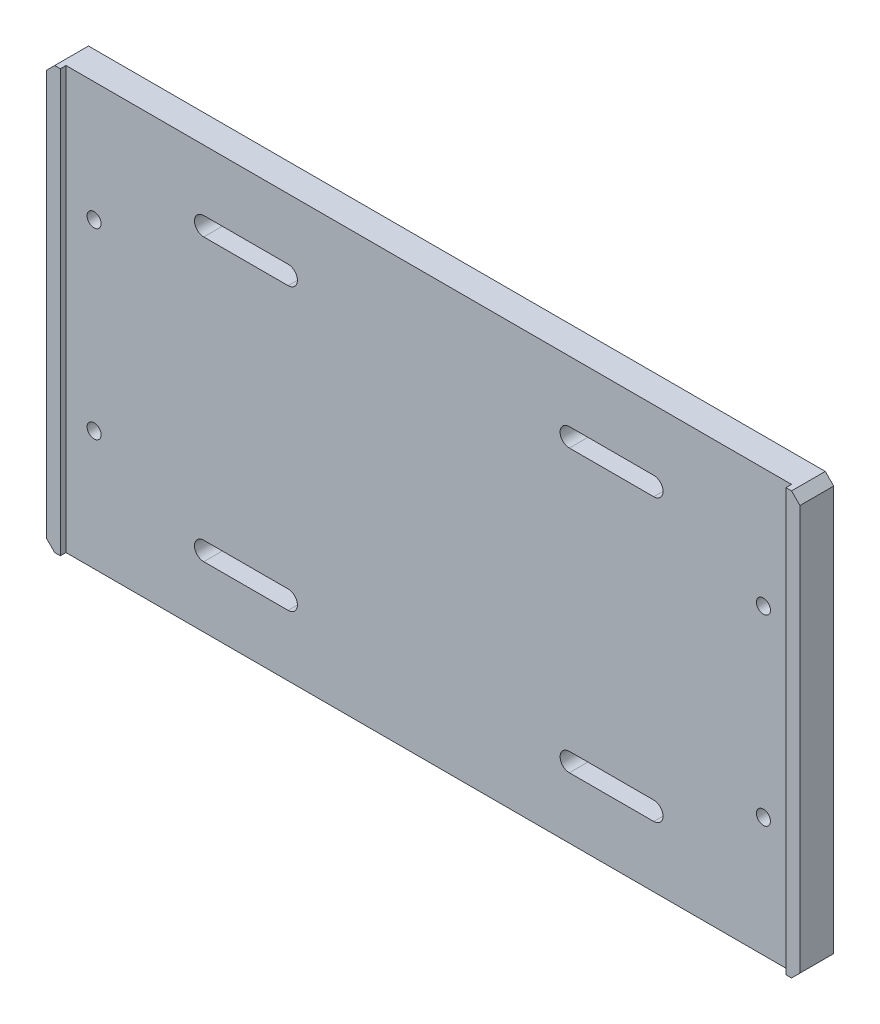
SolidWorks part; units mm, degrees
ref_plane "前视基准面" through (0, 0, 0) normal (0, 0, 1) x (1, 0, 0)
ref_plane "上视基准面" through (0, 0, 0) normal (0, 1, 0) x (1, 0, 0)
ref_plane "右视基准面" through (0, 0, 0) normal (1, 0, 0) x (0, 0, -1)
sketch "草图1" plane through (0, 0, 0) normal (0, 0, 1) x (1, 0, 0)
  line L1 (-134, -75) -> (134, -75)
  line L2 (-134, -75) -> (-134, 75)
  line L3 (-134, 75) -> (134, 75)
  line L4 (134, -75) -> (134, 75)
  line L5 (-134, -75) -> (134, 75) construction
  line L6 (-134, 75) -> (134, -75) construction
  point P0 (0, 0)
  dimension "D1" = 268
  dimension "D2" = 150
extrude "凸台-拉伸1" add sketch "草图1" along normal blind 12
sketch "草图2" plane through (0, 0, 12) normal (0, 0, 1) x (1, 0, 0)
  line L0 (134, 75) -> (-134, 75) construction
  line L1 (-129, -75) -> (129, -75)
  line L2 (-129, -75) -> (-129, 75)
  line L3 (-129, 75) -> (129, 75)
  line L4 (129, -75) -> (129, 75)
  line L5 (-129, -75) -> (129, 75) construction
  line L6 (-129, 75) -> (129, -75) construction
  line L7 (134, -75) -> (134, 75) construction
  point P0 (0, 0)
  dimension "D1" = 5
extrude "切除-拉伸1" cut sketch "草图2" against normal blind 2
sketch "草图3" plane through (0, 0, 10) normal (0, 0, 1) x (1, 0, 0)
  line L0 (-80, 50) -> (-50, 50) construction
  line L1 (-80, 53.3) -> (-50, 53.3)
  line L2 (-80, 46.7) -> (-50, 46.7)
  line L3 (50, 50) -> (80, 50) construction
  line L4 (50, 53.3) -> (80, 53.3)
  line L5 (50, 46.7) -> (80, 46.7)
  line L6 (-80, -50) -> (-50, -50) construction
  line L7 (-80, -46.7) -> (-50, -46.7)
  line L8 (-80, -53.3) -> (-50, -53.3)
  line L9 (50, -50) -> (80, -50) construction
  line L10 (50, -46.7) -> (80, -46.7)
  line L11 (50, -53.3) -> (80, -53.3)
  line L12 (0, 0) -> (0, 75) construction
  line L13 (129, 75) -> (-129, 75) construction
  line L14 (0, 0) -> (134, 0) construction
  line L15 (134, -75) -> (134, 75) construction
  arc A0 (-80, 53.3) -> (-80, 46.7) centre (-80, 50) ccw
  arc A1 (-50, 46.7) -> (-50, 53.3) centre (-50, 50) ccw
  arc A2 (50, 53.3) -> (50, 46.7) centre (50, 50) ccw
  arc A3 (80, 46.7) -> (80, 53.3) centre (80, 50) ccw
  arc A4 (-80, -46.7) -> (-80, -53.3) centre (-80, -50) ccw
  arc A5 (-50, -53.3) -> (-50, -46.7) centre (-50, -50) ccw
  arc A6 (50, -46.7) -> (50, -53.3) centre (50, -50) ccw
  arc A7 (80, -53.3) -> (80, -46.7) centre (80, -50) ccw
  point P2 (-65, 50)
  point P7 (65, 50)
  point P14 (-65, -50)
  point P21 (65, -50)
  dimension "D1" = 6.6
  dimension "D2" = 30
  dimension "D3" = 100
  dimension "D4" = 130
extrude "切除-拉伸2" cut sketch "草图3" against normal through all
hole_wizard "M6 螺纹孔1" positions "草图4" profile "草图5" tap size "M6" standard "ISO" end condition through all
sketch "草图4" plane through (0, 0, 10) normal (0, 0, 1) x (1, 0, 0)
  line L0 (0, 0) -> (0, 75) construction
  line L1 (129, 75) -> (-129, 75) construction
  line L3 (0, 0) -> (-129, 0) construction
  line L4 (-129, 75) -> (-129, -75) construction
  point P0 (-119, 32.5)
  point P2 (-119, -32.5)
  point P4 (119, 32.5)
  point P6 (119, -32.5)
  dimension "D1" = 65
  dimension "D2" = 238
sketch "草图5" plane through (-119, 32.5, 10) normal (1, 0, 0) x (0, -1, 0)
  line L0 (0, 0) -> (0, 10)
  line L1 (0, 10) -> (2.5, 10)
  line L2 (2.5, 10) -> (2.5, 0)
  line L5 (2.5, 0) -> (0, 0)
  line L11 (0, -6.35) -> (0, 107.95) construction
  dimension "通孔螺纹孔钻头直径" = 5
  dimension "通孔螺纹孔钻头深度" = 10
cosmetic thread "孔螺蚊线1" parameters "D2"=6
cosmetic thread "孔螺蚊线2" parameters "D2"=6
cosmetic thread "孔螺蚊线3" parameters "D2"=6
cosmetic thread "孔螺蚊线4" parameters "D2"=6
chamfer "倒角1" distance 3 angle 45 4 edges at (-134, 75, 6) (134, 75, 6) (134, -75, 6) (-134, -75, 6)
